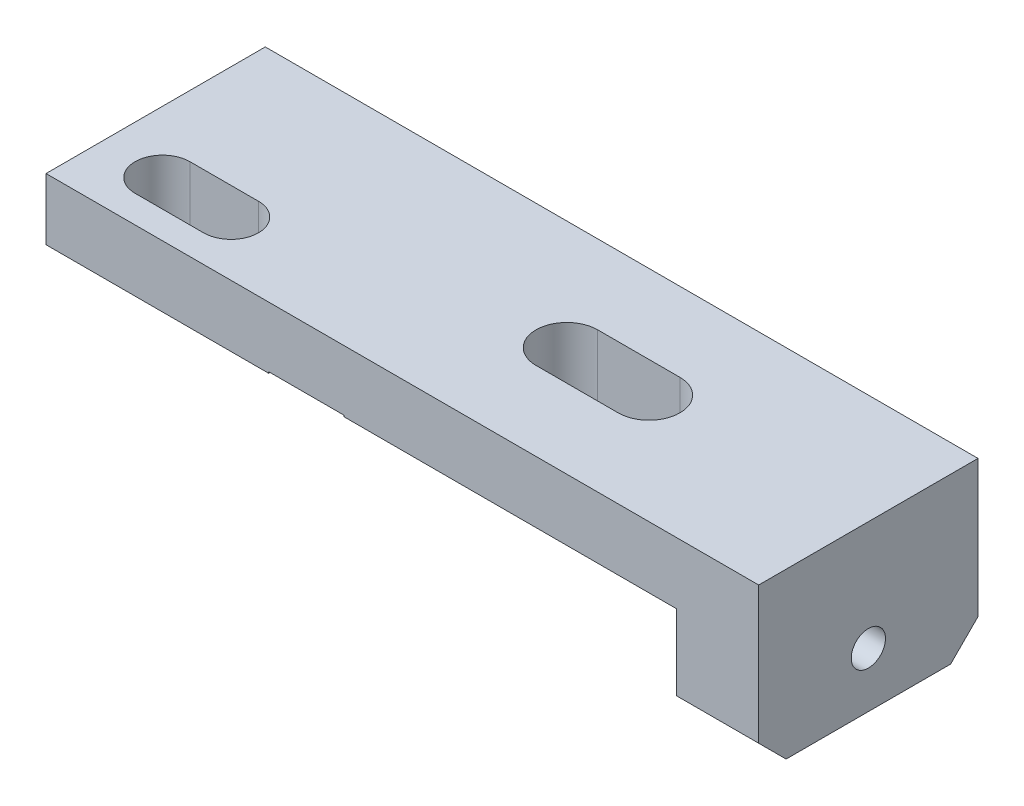
from build123d import *

# Parameters (mm, degrees)
SKETCH1_W             = 46
SKETCH1_H             = 16
BOSS_EXTRUDE1_DEPTH   = 4.5
SKETCH2_W             = 16
SKETCH2_H             = 12
BOSS_EXTRUDE2_DEPTH   = 6
SKETCH3_R             = 1
CUT_EXTRUDE1_DEPTH    = 10
M3_TAPPED_HOLE1_D     = 2.5
M3_TAPPED_HOLE1_DEPTH = 7.5
M3_TAPPED_HOLE1_TIP   = 0.751075774
CHAMFER1_SIZE         = 2
CUT_EXTRUDE2_DEPTH    = 7.5
CUT_EXTRUDE3_DEPTH    = 2.75
FILLET1_R             = 3
FILLET2_R             = 2
CUT_EXTRUDE4_DEPTH    = 15
CUT_EXTRUDE5_DEPTH    = 15
CHAMFER2_SIZE         = 0.5


with BuildPart() as part:
    # Sketch1 → Boss-Extrude1 (new body)
    with BuildSketch(Plane(origin=(0, 0, 0), x_dir=(1, 0, 0), z_dir=(0, 1, 0))):
        Rectangle(SKETCH1_W, SKETCH1_H)
    extrude(amount=BOSS_EXTRUDE1_DEPTH)

    # Sketch2 → Boss-Extrude2 (add)
    with BuildSketch(Plane(origin=(23, 0, 0), x_dir=(0, 0, -1), z_dir=(1, 0, 0))):
        with Locations((0, -1.5)):
            Rectangle(SKETCH2_W, SKETCH2_H)
    extrude(amount=BOSS_EXTRUDE2_DEPTH)

    # Sketch3 → Cut-Extrude1 (cut)
    with BuildSketch(Plane(origin=(29, 0, 0), x_dir=(0, 0, -1), z_dir=(1, 0, 0))):
        with Locations((0, -3.5)):
            Circle(SKETCH3_R)
    extrude(amount=-CUT_EXTRUDE1_DEPTH, mode=Mode.SUBTRACT)

    # M3 Tapped Hole1
    with Locations(Plane(origin=(29, -3.5, 0), x_dir=(0, 0, 1), z_dir=(1, 0, 0))):
        with Locations((0, 0)):
            Hole(M3_TAPPED_HOLE1_D / 2, depth=M3_TAPPED_HOLE1_DEPTH)
            with Locations((0, 0, -(M3_TAPPED_HOLE1_DEPTH + M3_TAPPED_HOLE1_TIP / 2))):  # 118° drill point
                Cone(0, M3_TAPPED_HOLE1_D / 2, M3_TAPPED_HOLE1_TIP, mode=Mode.SUBTRACT)

    # Chamfer1
    chamfer1_edges = [part.edges().sort_by_distance(p)[0] for p in [
        (26, -7.5, -8),
        (26, -7.5, 8),
    ]]
    chamfer(chamfer1_edges, length=CHAMFER1_SIZE)

    # Sketch5 → Cut-Extrude2 (cut, symmetric)
    with BuildSketch(Plane.ZY.offset(5.5)):
        Polygon((-1.4, 0), (-15.004762523, 0), (-15.004762523, 2.891781544), align=None)
    extrude(amount=CUT_EXTRUDE2_DEPTH, both=True, mode=Mode.SUBTRACT)

    # Sketch6 → Cut-Extrude3 (cut, symmetric)
    with BuildSketch(Plane.ZY.offset(4)):
        Polygon((-1.389489576, 0.1), (-8, 1.505107367), (-8, -0.5), (8, -0.5), (8, 0.1), align=None)
    extrude(amount=CUT_EXTRUDE3_DEPTH, both=True, mode=Mode.SUBTRACT)

    # Fillet1
    fillet1_edges = [part.edges().sort_by_distance(p)[0] for p in [
        (-4, 1.505107367, -8),
    ]]
    fillet(fillet1_edges, radius=FILLET1_R)

    # Fillet2
    fillet2_edges = [part.edges().sort_by_distance(p)[0] for p in [
        (-4, 0.1, -1.389489576),
    ]]
    fillet(fillet2_edges, radius=FILLET2_R)

    # Sketch7 → Cut-Extrude4 (cut)
    with BuildSketch(Plane(origin=(0, 4.5, 0), x_dir=(1, 0, 0), z_dir=(0, 1, 0))):
        with BuildLine():
            Line((-18.5, -2), (-13.5, -2))
            ThreePointArc((-13.5, -2), (-11.5, -4), (-13.5, -6))
            Line((-13.5, -6), (-18.5, -6))
            ThreePointArc((-18.5, -6), (-20.5, -4), (-18.5, -2))
        make_face()
    extrude(amount=-CUT_EXTRUDE4_DEPTH, mode=Mode.SUBTRACT)

    # Sketch8 → Cut-Extrude5 (cut)
    with BuildSketch(Plane(origin=(0, 4.5, 0), x_dir=(1, 0, 0), z_dir=(0, 1, 0))):
        with BuildLine():
            Line((7, 2.25), (13, 2.25))
            ThreePointArc((13, 2.25), (15.25, 0), (13, -2.25))
            Line((13, -2.25), (7, -2.25))
            ThreePointArc((7, -2.25), (4.75, 0), (7, 2.25))
        make_face()
    extrude(amount=-CUT_EXTRUDE5_DEPTH, mode=Mode.SUBTRACT)

    # Chamfer2
    chamfer2_edges = [part.edges().sort_by_distance(p)[0] for p in [
        (-1.25, 2.668666387, -8),
        (-6.75, 2.668666387, -8),
    ]]
    chamfer(chamfer2_edges, length=CHAMFER2_SIZE)


solid = part.part
